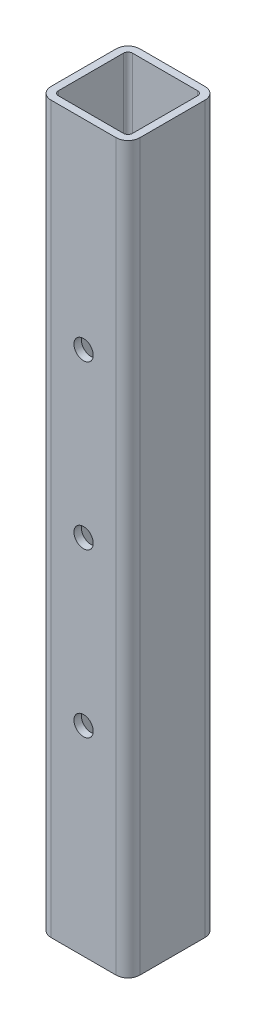
SolidWorks part; units mm, degrees
material "XRAAT"
ref_plane "前视基准面" through (0, 0, 0) normal (0, 0, 1) x (1, 0, 0)
ref_plane "上视基准面" through (0, 0, 0) normal (0, 1, 0) x (1, 0, 0)
ref_plane "右视基准面" through (0, 0, 0) normal (1, 0, 0) x (0, 0, -1)
sketch "草图1" plane through (0, 0, 0) normal (0, 0, 1) x (1, 0, 0)
  line L0 (0, 0) -> (0, 980)
  dimension "D1" = 980
other "结构用冷弯空心方钢(gb t6728-2002) 120×120×10(1)"
ref_plane "基准面1" through (0, 0, 0) normal (0, 1, 0) x (-1, 0, 0)
sketch "Sketch12" plane through (0, 0, 0) normal (0, 1, 0) x (-1, 0, 0)
  line L0 (-44, -50) -> (44, -50)
  line L1 (-50, -44) -> (-50, 44)
  line L2 (44, 50) -> (-44, 50)
  line L3 (50, 44) -> (50, -44)
  line L4 (-44, -60) -> (44, -60)
  line L5 (-60, -44) -> (-60, 44)
  line L6 (44, 60) -> (-44, 60)
  line L7 (60, 44) -> (60, -44)
  arc A0 (60, 44) -> (44, 60) centre (44, 44) ccw
  arc A1 (44, -60) -> (60, -44) centre (44, -44) ccw
  arc A2 (-60, -44) -> (-44, -60) centre (-44, -44) ccw
  arc A3 (-44, 60) -> (-60, 44) centre (-44, 44) ccw
  arc A4 (-44, 50) -> (-50, 44) centre (-44, 44) ccw
  arc A5 (50, 44) -> (44, 50) centre (44, 44) ccw
  arc A6 (44, -50) -> (50, -44) centre (44, -44) ccw
  arc A7 (-50, -44) -> (-44, -50) centre (-44, -44) ccw
  point P0 (-60, 0)
  point P1 (60, 0)
  point P2 (0, 60)
  point P3 (0, -60)
  point P4 (0, 0)
  point P5 (-60, -60)
  point P6 (60, -60)
  point P7 (60, 60)
  point P8 (-60, 60)
  point P33 (0, 0)
  dimension "D1" = 16
  dimension "D2" = 120
  dimension "D3" = 10
hole_wizard "Ø26 直径孔1" positions "草图2" profile "草图3" hole size "Ø12.0" standard "GB"
sketch "草图2" plane through (0, 0, 60) normal (0, 0, 1) x (1, 0, 0)
  line L0 (60, 490) -> (-60, 490) construction
  line L1 (60, 980) -> (60, 0) construction
  line L2 (-60, 980) -> (-60, 0) construction
  point P0 (0, 710)
  point P10 (0, 490)
  point P13 (0, 270)
  dimension "D1" = 440
sketch "草图3" plane through (0, 710, 60) normal (1, 0, 0) x (0, -1, 0)
  line L0 (0, 0) -> (0, 127.8102)
  line L1 (0, 127.8102) -> (13, 119.999)
  line L2 (13, 119.999) -> (13, 0)
  line L5 (13, 0) -> (0, 0)
  line L10 (0, 127.8102) -> (-13, 119.999) construction
  line L11 (0, -6.35) -> (0, 107.95) construction
  dimension "孔直径" = 26
  dimension "孔深度" = 119.999
  dimension "导头角度" = 118
